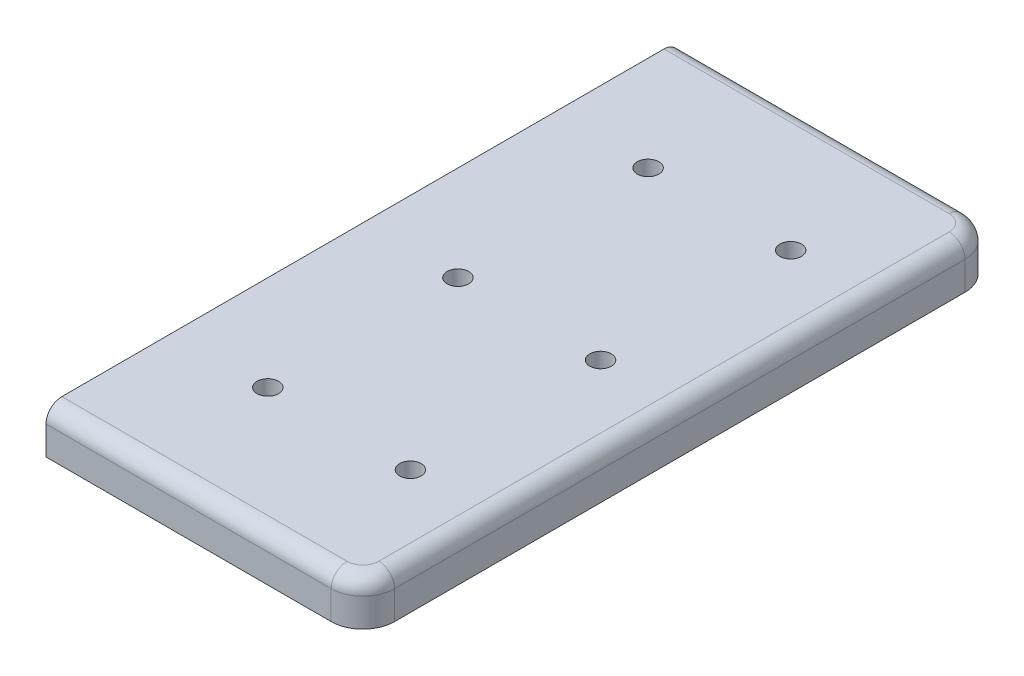
from build123d import *

# Parameters (mm, degrees)
SKETCH1_W                  = 100
SKETCH1_H                  = 200
BOSS_EXTRUDE1_DEPTH        = 14
FILLET1_R                  = 10
FILLET2_R                  = 5
SKETCH10_W                 = 40
SKETCH10_H                 = 150
BOSS_EXTRUDE3_DEPTH        = 3
SKETCH11_W                 = 10
SKETCH11_H                 = 150
CUT_EXTRUDE5_DEPTH         = 3
SKETCH12_W                 = 40
SKETCH12_H                 = 150
SKETCH12_W_2               = 30
CUT_EXTRUDE6_DEPTH         = 10
M8_TAPPED_HOLE2_AT_2_COUNT = 2
M8_TAPPED_HOLE2_AT_2_PITCH = 60
M8_TAPPED_HOLE2_AT_3_COUNT = 2
M8_TAPPED_HOLE2_AT_3_PITCH = 120
LPATTERN1_COUNT            = 2
LPATTERN1_PITCH            = 45
FILLET3_R                  = 5


with BuildPart() as part:
    # Sketch1 → Boss-Extrude1 (new body)
    with BuildSketch(Plane(origin=(0, 0, 0), x_dir=(1, 0, 0), z_dir=(0, 1, 0))):
        Rectangle(SKETCH1_W, SKETCH1_H)
    extrude(amount=BOSS_EXTRUDE1_DEPTH)

    # Fillet1
    fillet1_edges = [part.edges().sort_by_distance(p)[0] for p in [
        (50, 7, 100),
        (50, 7, -100),
    ]]
    fillet(fillet1_edges, radius=FILLET1_R)

    # Fillet2
    fillet2_edges = [part.edges().sort_by_distance(p)[0] for p in [
        (-5, 14, -100),
        (50, 14, 0),
        (-5, 14, 100),
        (47.071067812, 14, 97.071067812),
        (47.071067812, 14, -97.071067812),
    ]]
    fillet(fillet2_edges, radius=FILLET2_R)

    # Sketch10 → Boss-Extrude3 (add)
    with BuildSketch(Plane.XZ):
        with Locations((-25, 0)):
            Rectangle(SKETCH10_W, SKETCH10_H)
        with Locations((25, 0)):
            Rectangle(SKETCH10_W, SKETCH10_H)
    extrude(amount=BOSS_EXTRUDE3_DEPTH)

    # Sketch11 → Cut-Extrude5 (cut)
    with BuildSketch(Plane.XZ.offset(3)):
        with Locations((-40, 0)):
            Rectangle(SKETCH11_W, SKETCH11_H)
    extrude(amount=-CUT_EXTRUDE5_DEPTH, mode=Mode.SUBTRACT)

    # Sketch12 → Cut-Extrude6 (cut)
    with BuildSketch(Plane.XZ.offset(3)):
        with Locations((25, 0)):
            Rectangle(SKETCH12_W, SKETCH12_H)
        with Locations((-20, 0)):
            Rectangle(SKETCH12_W_2, SKETCH12_H)
    extrude(amount=-CUT_EXTRUDE6_DEPTH, mode=Mode.SUBTRACT)

    # Sketch14 → M8 Tapped Hole2 (revolve, cut)
    with BuildSketch(Plane(origin=(25, 7, -60), x_dir=(0, 0, -1), z_dir=(1, 0, 0))):
        Polygon((0, 0), (0, 21.792926105), (3.4, 19.75), (3.4, 0), align=None)
    m8_tapped_hole2 = revolve(axis=Axis((25, 0.65, -60), (0, 1, 0)), mode=Mode.SUBTRACT)

    # M8 Tapped Hole2 at 2: M8 Tapped Hole2 ×2
    with Locations(*[(0, 0, i * M8_TAPPED_HOLE2_AT_2_PITCH) for i in range(1, M8_TAPPED_HOLE2_AT_2_COUNT)]):
        add(m8_tapped_hole2, mode=Mode.SUBTRACT)

    # M8 Tapped Hole2 at 3: M8 Tapped Hole2 ×2
    with Locations(*[(0, 0, i * M8_TAPPED_HOLE2_AT_3_PITCH) for i in range(1, M8_TAPPED_HOLE2_AT_3_COUNT)]):
        add(m8_tapped_hole2, mode=Mode.SUBTRACT)

    # LPattern1: M8 Tapped Hole2 ×2
    with Locations(*[(-i * LPATTERN1_PITCH, 0, 0) for i in range(1, LPATTERN1_COUNT)]):
        add(m8_tapped_hole2, mode=Mode.SUBTRACT)

    # LPattern1 copy 1 sketch → LPattern1 copy 1 (revolve, cut)
    with BuildSketch(Plane(origin=(-20, 7, 0), x_dir=(0, 0, -1), z_dir=(1, 0, 0))):
        Polygon((0, 0), (0, 21.792926105), (3.4, 19.75), (3.4, 0), align=None)
    revolve(axis=Axis((-20, 0.65, 0), (0, 1, 0)), mode=Mode.SUBTRACT)

    # LPattern1 copy 2 sketch → LPattern1 copy 2 (revolve, cut)
    with BuildSketch(Plane(origin=(-20, 7, 60), x_dir=(0, 0, -1), z_dir=(1, 0, 0))):
        Polygon((0, 0), (0, 21.792926105), (3.4, 19.75), (3.4, 0), align=None)
    revolve(axis=Axis((-20, 0.65, 60), (0, 1, 0)), mode=Mode.SUBTRACT)

    # Fillet3
    fillet3_edges = [part.edges().sort_by_distance(p)[0] for p in [
        (45, 3.5, 75),
        (45, 3.5, -75),
        (5, 3.5, -75),
        (5, 3.5, 75),
        (-5, 3.5, 75),
        (-35, 3.5, -75),
        (-35, 3.5, 75),
        (-5, 3.5, -75),
    ]]
    fillet(fillet3_edges, radius=FILLET3_R)


solid = part.part
